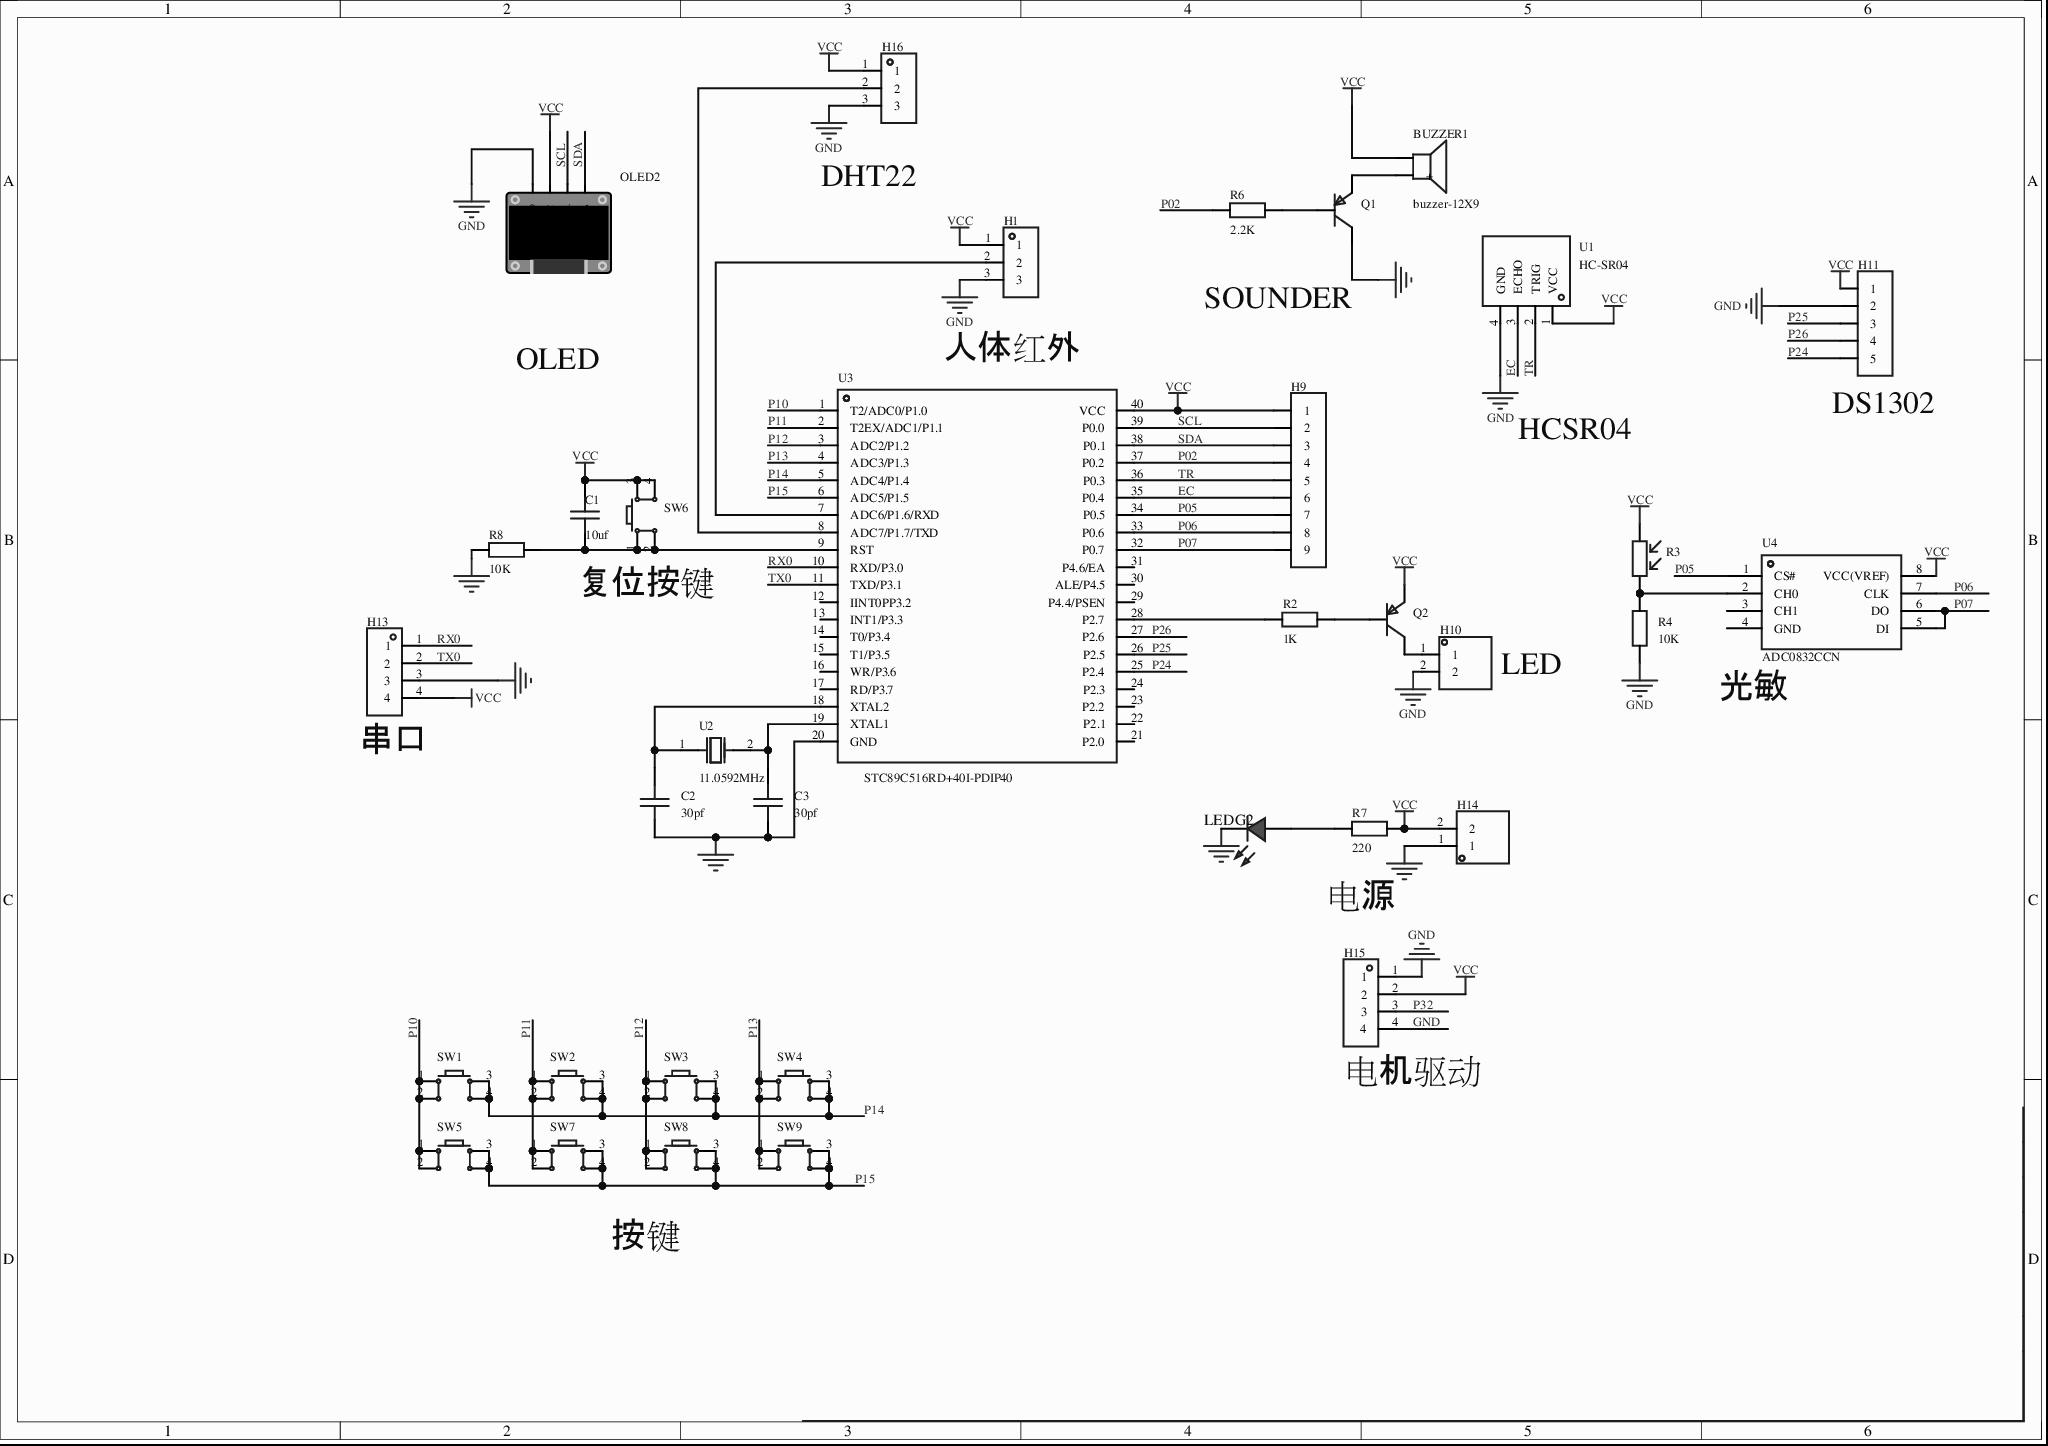
[diagram p0: MISC52077-3.schdoc]
# Altium project MISC52077-2.PrjPcb
1 sheet, 35 parts. Net scope: global (net labels, ports and power ports of the same name join across sheets).
Board file: MISC52077.pcbdoc

## Sheet MISC52077-3.schdoc
size 297 x 209 mm; Version: V1.0; @Project Name: MISC52077; @Page Count: 1; @Update Date: 2026-04-26; @Create Date: 2026-04-26; @Schematic Name: MISC52077; @Page No: 1; @Create Time: 23:22:16; @Update Time: 17:32:40; @Board Name: MISC52077

### Parts
BUZZER1  buzzer-12X9  [BUZ-TH_BD12.0-P7.60-D0.6-FD]
C1  10uf  [C0805]
C2  30pf  [C0805]
C3  30pf  [C0805]
H1  (no value)  [HDR-TH_3P-P2.54-V-F]
H9  (no value)  [HDR-TH_9P-P2.54-V-F-1]
H10  (no value)  [HDR-TH_2P-P2.54-V-M-1]
H11  (no value)  [HDR-TH_5P-P2.54-V-F]
H13  (no value)  [HDR-TH_4P-P2.54-V-M]
H14  (no value)  [HDR-TH_2P-P2.54-V-M-1]
H15  (no value)  [HDR-TH_4P-P2.54-V-F]
H16  (no value)  [HDR-TH_3P-P2.54-V-F]
LEDG2  (no value)  [LED_0805]
OLED2  (no value)  [0.96OLED_4P]
Q1  2N3906S-RTK/PS  [SOT-23-3_L2.9-W1.3-P1.90-LS2.4-TR]  (value not drawn)
Q2  (no value)  [S8550P_SOT]
R2  1K  [R0805]
R3  GL5549(80-100)  [RES-TH_L5.1-W4.3-P3.40-D0.5]  (value not drawn)
R4  10K  [R0805]
R6  2.2K  [R0805]
R7  220  [R0805]
R8  10K  [R0805]
SW1  (no value)  [SW-TH_4P-L6.0-W6.0-P4.50-LS6.5]
SW2  (no value)  [SW-TH_4P-L6.0-W6.0-P4.50-LS6.5]
SW3  (no value)  [SW-TH_4P-L6.0-W6.0-P4.50-LS6.5]
SW4  (no value)  [SW-TH_4P-L6.0-W6.0-P4.50-LS6.5]
SW5  (no value)  [SW-TH_4P-L6.0-W6.0-P4.50-LS6.5]
SW6  (no value)  [SW-TH_4P-L6.0-W6.0-P4.50-LS6.5]
SW7  (no value)  [SW-TH_4P-L6.0-W6.0-P4.50-LS6.5]
SW8  (no value)  [SW-TH_4P-L6.0-W6.0-P4.50-LS6.5]
SW9  (no value)  [SW-TH_4P-L6.0-W6.0-P4.50-LS6.5]
U1  HC-SR04  [TH_HC-SR04V]
U2  11.0592MHz  [HC-49US_L11.0-W4.6-P4.88]
U3  STC89C516RD+40I-PDIP40  [DIP-40_L52.3-W13.9-P2.54-LS15.2-BL]
U4  ADC0832CCN  [DIP-8_L9.7-W6.4-P2.54-LS7.6-BL]

### Nets
GND: C2.1 C3.1 H1.3 H10.2 H11.2 H13.3 H14.1 H15.1 H15.4 H16.3 LEDG2.1(C) OLED2.1(GND) Q1.3(C) R4.1 R8.2 U1.4(GND) U3.20(GND)
VCC: BUZZER1.2 C1.2 H1.1 H9.1 H11.1 H13.4 H14.2 H15.2 H16.1 OLED2.2(VCC) Q2.2(E) R3.1 R7.2 SW6.3 SW6.4 U1.1(VCC) U3.40(VCC) U4.8(VCC(VREF))
EC: H9.6 U1.3(ECHO) U3.35(P0.4)
P02: H9.4 R6.1 U3.37(P0.2)
P05: H9.7 U3.34(P0.5) U4.1(CS#)
P06: H9.8 U3.33(P0.6) U4.7(CLK)
P07: H9.9 U3.32(P0.7) U4.5(DI) U4.6(DO)
P10: SW1.1 SW1.2 SW5.1 SW5.2 U3.1(T2/ADC0/P1.0)
P11: SW2.1 SW2.2 SW7.1 SW7.2 U3.2(T2EX/ADC1/P1.1)
P12: SW3.1 SW3.2 SW8.1 SW8.2 U3.3(ADC2/P1.2)
P13: SW4.1 SW4.2 SW9.1 SW9.2 U3.4(ADC3/P1.3)
P14: SW1.3 SW1.4 SW2.3 SW2.4 SW3.3 SW3.4 SW4.3 SW4.4 U3.5(ADC4/P1.4)
P15: SW5.3 SW5.4 SW7.3 SW7.4 SW8.3 SW8.4 SW9.3 SW9.4 U3.6(ADC5/P1.5)
P24: H11.5 U3.25(P2.4)
P25: H11.3 U3.26(P2.5)
P26: H11.4 U3.27(P2.6)
P32: H15.3
RX0: H13.1 U3.10(RXD/P3.0)
SCL: H9.2 OLED2.3(SCL) U3.39(P0.0)
SDA: H9.3 OLED2.4(SDA) U3.38(P0.1)
TR: H9.5 U1.2(TRIG) U3.36(P0.3)
TX0: H13.2 U3.11(TXD/P3.1)
NetBUZZER1_1: BUZZER1.1(+) Q1.1(E)
NetC1_1: C1.1 R8.1 SW6.1 SW6.2 U3.9(RST)
NetC2_2: C2.2 U2.1(OSC1) U3.18(XTAL2)
NetC3_2: C3.2 U2.2(OSC2) U3.19(XTAL1)
NetH1_2: H1.2 U3.7(ADC6/P1.6/RXD)
NetH10_1: H10.1 Q2.3(C)
NetH16_2: H16.2 U3.8(ADC7/P1.7/TXD)
NetLEDG2_2: LEDG2.2(A) R7.1
NetQ1_2: Q1.2(B) R6.2
NetQ2_1: Q2.1(B) R2.2
NetR2_1: R2.1 U3.28(P2.7)
NetR3_2: R3.2 R4.2 U4.2(CH0)

Not connected (* = marked no-connect by the designer): U3 12(IINT0PP3.2) 13(INT1/P3.3) 14(T0/P3.4) 15(T1/P3.5) 16(WR/P3.6) 17(RD/P3.7) 21(P2.0) 22(P2.1) 23(P2.2) 24(P2.3) 29(P4.4/PSEN) 30(ALE/P4.5) 31(P4.6/EA); U4 3(CH1) 4(GND)

### Notes on the sheet
- (near H16) DHT22
- SOUNDER
- OLED
- 人体红外
- (near H11) DS1302
- HCSR04
- 复位按键
- LED
- (near H13) 串口
- (near U4) 光敏
- 电源
- (near H15) 电机驱动
- 按键

### Library data of the parts
BUZZER1 = buzzer-12X9: 3D Model: 16ab50e14c5b4f2c986c135bdba60e37; 3D Model Transform: 472.44,472.176,0,90,0,0,-0.787,0,-177.165; AddInBom: yes; ModelName: BUZ-TH_D12.0-H9.5-P7.60; Symbol: BUZZER-12X9; Device: buzzer-12X9; LCSC Part Name: buzzer-12X9; Supplier Part: C9900016920; Manufacturer Part: buzzer-12X9; Supplier Footprint: BUZZER_SMT_9650B; JLCPCB Part Class: 扩展库; Supplier: LCSC; ConvertToPcb: yes; FootprintName: BUZ-TH_BD12.0-P7.60-D0.6-FD
C1-C3 = CAP_0805: Symbol: CapAcitance; 3D Model: 1ba041120af144c991958decab20d241; 3D Model Transform: 78.74,51.181,0,0,0,0,0,0.0005,0; ConvertToPcb: yes; ModelName: C0805_L2.0-W1.3-H1.3; Device: CAP_0805; Supplier Footprint: 0805; AddInBom: yes; FootprintName: C0805
  C1: Value: 10uf
  C2 C3: Value: 30pf
H1 H16 = HDR-F_2.54_1x3P: Symbol: PM254V-11-03-H85; ConvertToPcb: yes; ModelId: f3b3cc5aae9641bf9e56fc160cef875b; ModelName: HDR2.54-F-LI-1X3P; ModelTransform: 299.9994,100,0,0,0,0,0,0,-118.11; Device: HDR-F_2.54_1x3P; AddInBom: yes; SupplierPart: C541850; Supplier Footprint: 插件; FootprintName: HDR-TH_3P-P2.54-V-F
H9 = HDR-F_2.54_1x9P: Symbol: Header-Female-2.54_1x9; 3D Model: 3a7016416d904017ac5ead6cc0f14e9c; 3D Model Transform: 915.746,94.488,0,0,0,0,0,0,-125.984; AddInBom: yes; ModelName: HDR-TH_9P-P2.54-F-LI-1X9P; Device: HDR-F_2.54_1x9P; Supplier Part: C39576; Supplier Footprint: 插件; JLCPCB Part Class: 扩展库; ConvertToPcb: yes; FootprintName: HDR-TH_9P-P2.54-V-F-1
H10 H14 = HDR-M_2.54_1x2P: Symbol: 210S-1*2P L=11.6MMGold-plated black; 3D Model: 79b2e9f2d70a4d68a1b7098f27c6d4c5; 3D Model Transform: 200,100,0,0,0,0,0,0,-118.11; ConvertToPcb: yes; ModelName: HDR-M-2.54_1x2; Device: HDR-M_2.54_1x2P; Supplier Part: C124375; Supplier Footprint: 插件; AddInBom: yes; FootprintName: HDR-TH_2P-P2.54-V-M-1
H11 = HDR-F_2.54_1x5P: Symbol: Header-Female-2.54_1x5; 3D Model: f49cb6116a3d45e5a64915bf3e00773f; 3D Model Transform: 519.684,98.464,0,0,0,0,0,0,-124.016; ConvertToPcb: yes; Device: HDR-F_2.54_1x5P; Supplier Part: C50950; Supplier Footprint: 插件; AddInBom: yes; FootprintName: HDR-TH_5P-P2.54-V-F; ModelName: HDR-TH_5P-P2.54-V-F
H13 = HDR-M_2.54_1x4P: Symbol: PZ254V-11-04P; 3D Model: 112f4d05e8d64e99ab9a333894bea4f9; 3D Model Transform: 399.999,104.7242,0,0,0,0,0,0,-118.11; ConvertToPcb: yes; ModelName: HDR-TH_4P-P2.54-M-LI-1X4P; Device: HDR-M_2.54_1x4P; Supplier Part: C492403; Supplier Footprint: 插件; AddInBom: yes; FootprintName: HDR-TH_4P-P2.54-V-M
H15 = HDR-F_2.54_1x4P: Symbol: 2.54-1*4P母; ConvertToPcb: yes; ModelId: d187812051054f85879fcaa51a310d8e0819f05c4eef4c71ace90d822a990e87; ModelTransform: 419.6842,98.464,0,0,0,0,0,0,-118.11; Device: HDR-F_2.54_1x4P; AddInBom: yes; SupplierPart: C2718488; Supplier Footprint: 插件; FootprintName: HDR-TH_4P-P2.54-V-F; ModelName: HDR-TH_4P-P2.54-V-F
LEDG2 = LED_0805-R: Symbol: LED_R; Convert to PCB: yes; 3D Model: 33fb9fca58e84f37a403ebeef4c28b77; 3D Model Transform: 78.7,49.1,39.3,0,0,0,0,0,0; ModelName: LED-0805_R; Device: LED_0805-R; Add into BOM: yes; Supplier Footprint: 0805; FootprintName: LED_0805
OLED2 = 0.96OLED模块_4P: ConvertToPcb: yes; ModelId: 79c000fdb68d45a296c2e9bedf4f9055; ModelTransform: 1393.69792,1318.895,0,0,0,0,0,-560.079,-137.795; Symbol: 0.96OLED模块_4P; Device: 0.96OLED模块_4P; AddInBom: yes; FootprintName: 0.96OLED_4P; Supplier Footprint: 插件; ModelName: 0.96OLED_4P
Q1 = 2N3906S-RTK/PS: Manufacturer: KEC; Symbol: 2N3906S-RTK/PS_C5300004; 3D Model: c62791f0466c4ae2a892c056b845b0ca; 3D Model Transform: 98.64468,114.173,0,180,0,0,0,0,0; AddInBom: yes; ModelName: SOT-23-3P_L2.9-W1.3-H1.0-LS2.4-P0.95; Device: 2N3906S-RTK/PS; LCSC Part Name: 2N3906S-RTK/PS; Supplier Part: C5300004; Manufacturer Part: 2N3906S-RTK/PS; Supplier Footprint: SOT-23; JLCPCB Part Class: 扩展库; Datasheet: https://atta.szlcsc.com/upload/public/pdf/source/20210607/C2837301_49A1D1F6E48E358BFC68D493EE9D29A5.pdf; Supplier: LCSC; ConvertToPcb: yes; FootprintName: SOT-23-3_L2.9-W1.3-P1.90-LS2.4-TR
Q2 = S8550_SOT_PNP: Symbol: PNP; ConvertToPcb: yes; ModelId: 9c0df02d6f3e44e889da37f3e5bf54960819f05c4eef4c71ace90d822a990e87; ModelName: SOT-23-3_L2.9-W1.4-P1.90-LS2.5-BR; ModelTransform: 98.43,114.17,37.91,0,0,0,0,0,0; Device: S8550_SOT_PNP; AddInBom: yes; Supplier Footprint: SOT-23; FootprintName: S8550P_SOT
R2 R4 R6-R8 = Res_0805: Symbol: 电阻; 3D Model: 37a81e68749a4138bd2dfa6897b24b85; 3D Model Transform: 78.74,51.181,0,0,0,0,0,-0.0005,0; ConvertToPcb: yes; ModelName: R0805_L2.0-W1.3-H0.6; Device: Res_0805; Supplier Footprint: 0805; AddInBom: yes; FootprintName: R0805
  R2: Value: 1K
  R4 R8: Value: 10K
  R6: Value: 2.2K
  R7: Value: 220
R3 = GL5549(80-100): 暗电阻:20MΩ;亮电阻@10Lux:80kΩ~150kΩ;光谱峰值(波长):540nm;; Manufacturer: JCHL(晶创和立); AddInBom: yes; ModelId: cb75fcf2d6c94cac811f2579121b87200819f05c4eef4c71ace90d822a990e87; ModelTransform: 169.291,200.39669,0,0,0,0,-3.937,0,-137.795; Dark Resistance: 20MΩ; Voltage - Max: 150V; Wavelength - Peak: 540nm; γ Value: 0.8; Pitch: 3.4mm; Symbol: GL5549(80-100); Device: GL5549(80-100); LCSC Part Name: 光敏电阻性能参数; SupplierPart: C10078; ManufacturerPart: GL5549(80-100); Supplier Footprint: 插件,P=3.4mm; JLCPCB Part Class: Extended Part; Datasheet: https://item.szlcsc.com/datasheet/GL5549(80-100)/10617.html; Supplier: LCSC; ConvertToPcb: yes; FootprintName: RES-TH_L5.1-W4.3-P3.40-D0.5; ModelName: RES-TH_L5.1-W4.3-P3.40-D0.5; Cell Resistance @ Illuminance: 80kΩ~150kΩ; Operating Temperature: -30℃~+70℃; Length: 5.1mm; Width: 4.3mm; Height: 2.4mm
SW1-SW4 SW6 = Key_TH_6x6x6: 触点电流:50mA;额定电压(DC):12V;绝缘电阻:100MΩ;电路结构:单刀单掷;安装方式:直插;按钮形状:圆形按钮;按钮/盖帽颜色:黑色;作用力:260gf@±30gf;工作温度:-25℃~+70℃;引脚样式:PC引脚;开关长度:6mm;开关宽度:6mm;开关高度:6mm;带支架:否;; Symbol: 轻触按键; AddInBom: yes; ModelId: 20eee248bc684ccd8cbdbb1d0d91ec6f0819f05c4eef4c71ace90d822a990e87; ModelName: SW-TH_4P-L6.0-W6.0-H5.0-LS6.5-P4.50; ModelTransform: 236.22,323.03,0,90,0,0,0,0,-137.795; Device: Key_TH_6x6x6; FootprintName: SW-TH_4P-L6.0-W6.0-P4.50-LS6.5; ConvertToPcb: yes; Supplier Footprint: 插件
SW5 SW7-SW9 = Key_TH_6x6x6: 触点电流:50mA;额定电压(DC):12V;绝缘电阻:100MΩ;电路结构:单刀单掷;安装方式:直插;按钮形状:圆形按钮;按钮/盖帽颜色:黑色;作用力:260gf@±30gf;工作温度:-25℃~+70℃;引脚样式:PC引脚;开关长度:6mm;开关宽度:6mm;开关高度:6mm;带支架:否;; Symbol: 轻触按键; 3D Model: 20eee248bc684ccd8cbdbb1d0d91ec6f0819f05c4eef4c71ace90d822a990e87; 3D Model Transform: 236.22,323.03,0,90,0,0,0,0,-137.795; AddInBom: yes; ModelName: SW-TH_4P-L6.0-W6.0-H5.0-LS6.5-P4.50; Device: Key_TH_6x6x6; Supplier Footprint: 插件; FootprintName: SW-TH_4P-L6.0-W6.0-P4.50-LS6.5; ConvertToPcb: yes
U1 = HC-SR04: Manufacturer: Universal Microelectronics; AddInBom: yes; Symbol: HC-SR04; Device: HC-SR04; LCSC Part Name: HC-SR04; SupplierPart: C19857336; ManufacturerPart: HC-SR04; Supplier Footprint: -; JLCPCB Part Class: 扩展库; Datasheet: https://atta.szlcsc.com/upload/public/pdf/source/20240122/47B8E374E428935B7962A2189EF91AAC.pdf; Supplier: LCSC; ConvertToPcb: yes; FootprintName: TH_HC-SR04V
U2 = ECS-120-S-4: 频率:12MHz;常温频差:±30ppm;外接负载电容:-;频率稳定度(全温):±50ppm;; Manufacturer: ECS; 3D Model: 59d05c800eee432cb051aa4925461fda; 3D Model Transform: 432.44473,183.0705,0,0,0,0,0,0,-137.795; Normal temperature Frequency Tolerance: ±30ppm; Frequency Stability(Full temperature range): ±50ppm; Equivalent Series Resistance (ESR): 60Ω; AddInBom: yes; ModelName: HC-49US_L11.0-W4.7-H3.5-P4.88; Symbol: ECS-120-S-4; Device: ECS-120-S-4; Value: 11.0592MHz; LCSC Part Name: 12MHz ±30ppm; Manufacturer Part: ECS-120-S-4; Supplier Footprint: HC-49S; JLCPCB Part Class: 扩展库; Datasheet: https://atta.szlcsc.com/upload/public/pdf/source/20210402/81F084B668D60DFAE850A61100CCABAF.pdf; Supplier: LCSC; External load capacitor: -; Operating Temperature: -10℃~+70℃; ConvertToPcb: yes; FootprintName: HC-49US_L11.0-W4.6-P4.88
U3 = STC89C516RD+40I-PDIP40: CPU内核:51系列;程序存储容量:61KB;RAM总容量:1.25KB;GPIO端口数量:35;工作电压范围:3.5V~5.5V;CPU最大主频:-;程序存储器类型:FLASH;; Manufacturer: STC(宏晶); 3D Model: 16d4686a009b4ddca948f91eddb57b14; 3D Model Transform: 2059.051,615.743,0,0,0,0,0,0,-129.921; CPU Core: 51系列; Program Storage Size: 61KB; RAM Size: 1.25KB; GPIO Ports Number: 35; Program Memory Type: FLASH; 16Bit Timer: 3; UART/USART: 1; Peripheral/Function: 看门狗; Watchdog: 有; AddInBom: yes; ModelName: DIP-40_L52.3-W13.8-H4.0-LS15.24-P2.54; Symbol: STC89C516RD+40I-PDIP40; Device: STC89C516RD+40I-PDIP40; LCSC Part Name: STC89C516RD+40I-PDIP40; Supplier Part: C52225; Manufacturer Part: STC89C516RD+40I-PDIP40; Supplier Footprint: DIP-40; JLCPCB Part Class: 扩展库; Datasheet: https://atta.szlcsc.com/upload/public/pdf/source/20180614/C87831_BBAF7FB8B286C29ACE4E9B180C033FEC.pdf; Supplier: LCSC; Operating Voltage Range: 3.5V~5.5V; CPU Maximum Speed: -; Operating Temperature Range: -40℃~+85℃; ADC (Bit): -; DAC (Bit): -; PWM (Bit): -; 8Bit Timer: -; 32Bit Timer: -; CAN: -; I2C: -; I2S: -; SPI: -; Universal Serial Bus: -; Internal Comparator: -; communication protocol: -; Real-Time Clock: -; Infrared Data Association: -; Low-Voltage Detect: -; CCP Capture/Compare: -; Secure Digital Input and Output: -; Direct Memory Access: -; Internal Oscillator: -; ConvertToPcb: yes; FootprintName: DIP-40_L52.3-W13.9-P2.54-LS15.2-BL
U4 = ADC0832CCN: AddInBom: yes; ModelId: 5746b540d01a4d1b9eb6b4f989297bc70819f05c4eef4c71ace90d822a990e87; ModelName: DIP-8_L9.8-W6.6-H3.5-LS7.62-P2.54; ModelTransform: 385.826,311.8104,0,0,0,0,0,0,-118.11; Symbol: ADC0832CCN; Device: ADC0832CCN; LCSC Part Name: ADC0832CCN; SupplierPart: C10915; ManufacturerPart: ADC0832CCN; Supplier Footprint: DIP-8; JLCPCB Part Class: Extended Part; Supplier: LCSC; ConvertToPcb: yes; FootprintName: DIP-8_L9.7-W6.4-P2.54-LS7.6-BL